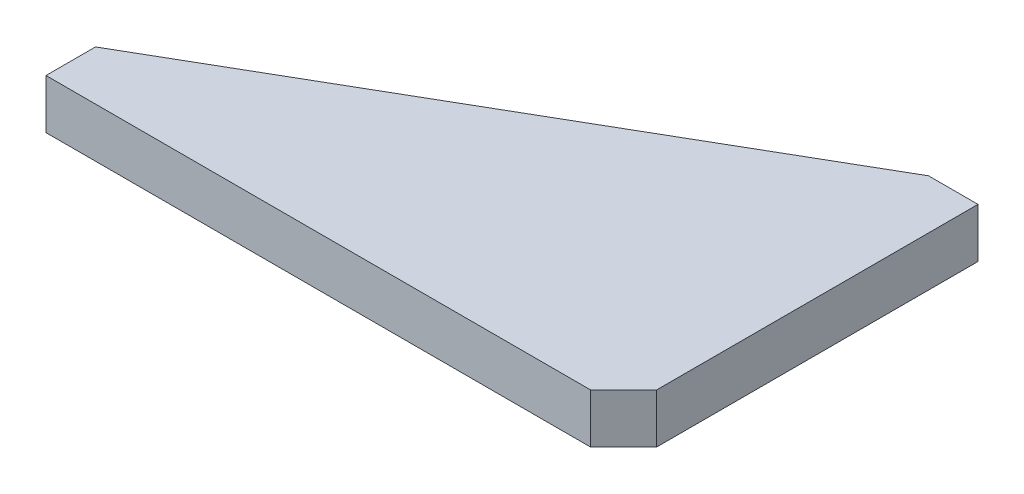
SolidWorks part; units mm, degrees
ref_plane "前视基准面" through (0, 0, 0) normal (0, 0, 1) x (1, 0, 0)
ref_plane "上视基准面" through (0, 0, 0) normal (0, 1, 0) x (1, 0, 0)
ref_plane "右视基准面" through (0, 0, 0) normal (1, 0, 0) x (0, 0, -1)
sketch "草图1" plane through (0, 0, 0) normal (0, 1, 0) x (1, 0, 0)
  line L0 (0, 0) -> (-30, 0)
  line L1 (-30, 0) -> (-350, -184.7521)
  line L2 (-350, -184.7521) -> (-350, -214.7521)
  line L3 (-350, -214.7521) -> (-20, -214.7521)
  line L4 (-20, -214.7521) -> (0, -194.7521)
  line L5 (0, -194.7521) -> (0, 0)
  dimension "D1" = 30
  dimension "D2" = 30
  dimension "D3" = 30
  dimension "D4" = 350
  dimension "D5" = 45
  dimension "D6" = 20
extrude "凸台-拉伸1" add sketch "草图1" along normal blind 30
